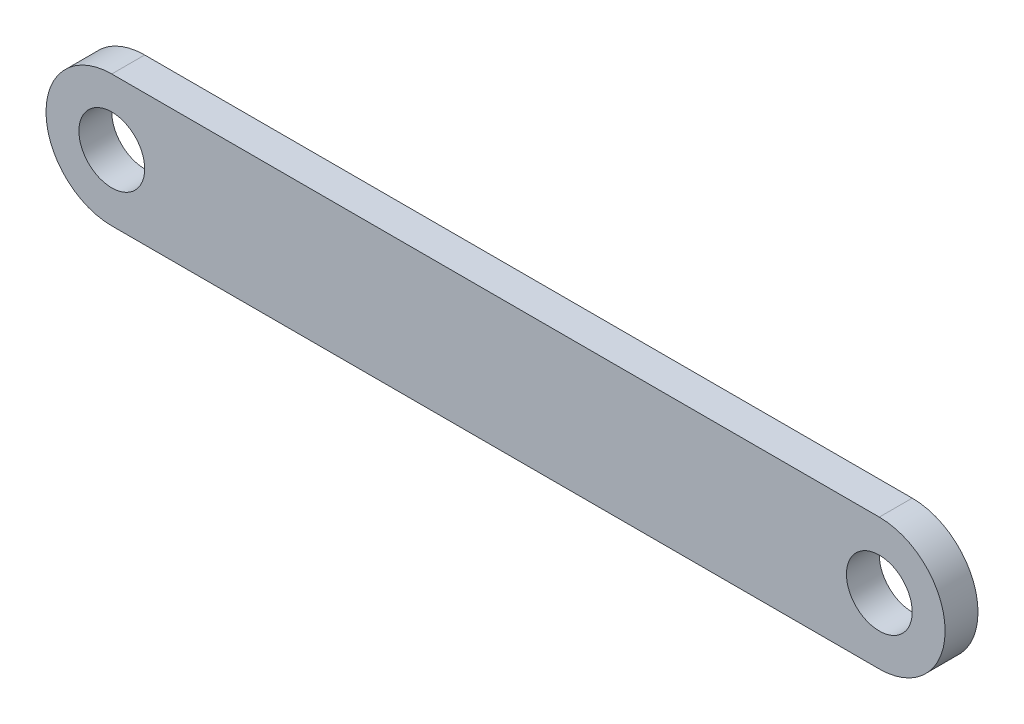
SolidWorks part; units mm, degrees
ref_plane "Front Plane" through (0, 0, 0) normal (0, 0, 1) x (1, 0, 0)
ref_plane "Top Plane" through (0, 0, 0) normal (0, 1, 0) x (1, 0, 0)
ref_plane "Right Plane" through (0, 0, 0) normal (1, 0, 0) x (0, 0, -1)
sketch "Sketch1" plane through (0, 0, 0) normal (0, 0, 1) x (1, 0, 0)
  line L0 (0, 0) -> (70, 0) construction
  line L1 (0, 6) -> (70, 6)
  line L2 (0, -6) -> (70, -6)
  arc A0 (0, 6) -> (0, -6) centre (0, 0) ccw
  arc A1 (70, -6) -> (70, 6) centre (70, 0) ccw
  circle A2 centre (0, 0) radius 3
  circle A3 centre (70, 0) radius 3
  point P3 (35, 0)
  dimension "D3" = 6
  dimension "D1" = 12
  dimension "D2" = 70
extrude "Boss-Extrude1" add sketch "Sketch1" along normal blind 3
